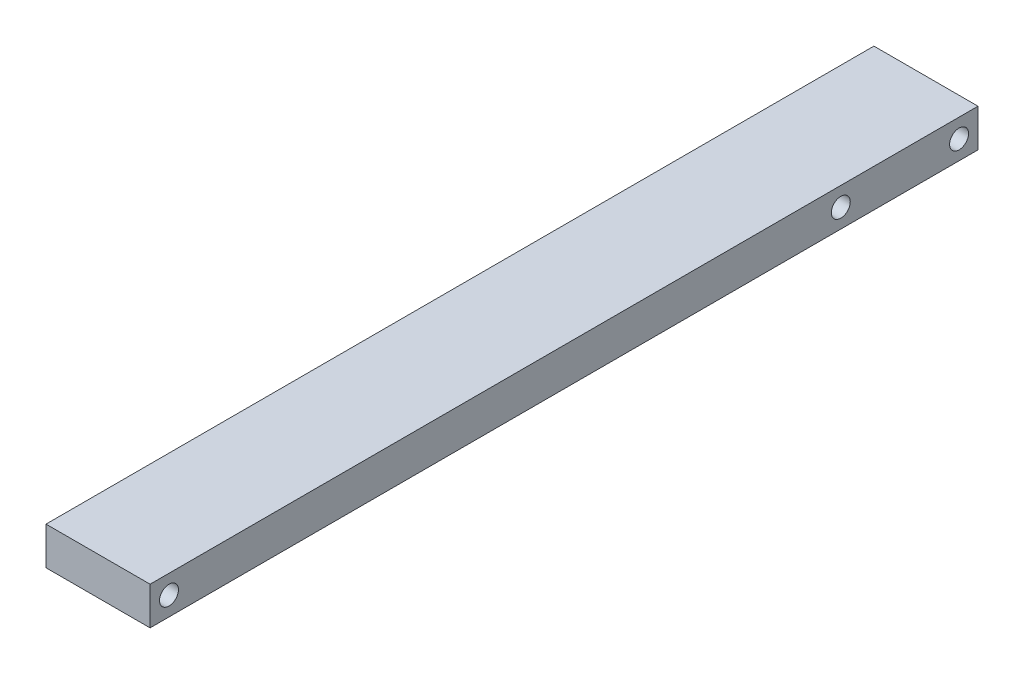
from build123d import *

# Parameters (mm, degrees)
SKETCH1_W           = 22
SKETCH1_H           = 8
BOSS_EXTRUDE1_DEPTH = 175
SKETCH2_R           = 2
CUT_EXTRUDE1_DEPTH  = 177.558772085


with BuildPart() as part:
    # Sketch1 → Boss-Extrude1 (new body)
    with BuildSketch(Plane.XY):
        with Locations((11, 4)):
            Rectangle(SKETCH1_W, SKETCH1_H)
    extrude(amount=BOSS_EXTRUDE1_DEPTH)

    # Sketch2 → Cut-Extrude1 (cut, through all)
    with BuildSketch(Plane(origin=(22, 0, 0), x_dir=(0, 0, -1), z_dir=(1, 0, 0))):
        with Locations((-4, 4)):
            Circle(SKETCH2_R)
        with Locations((-171, 4)):
            Circle(SKETCH2_R)
        with Locations((-29, 4)):
            Circle(SKETCH2_R)
    extrude(amount=-CUT_EXTRUDE1_DEPTH, mode=Mode.SUBTRACT)


solid = part.part
